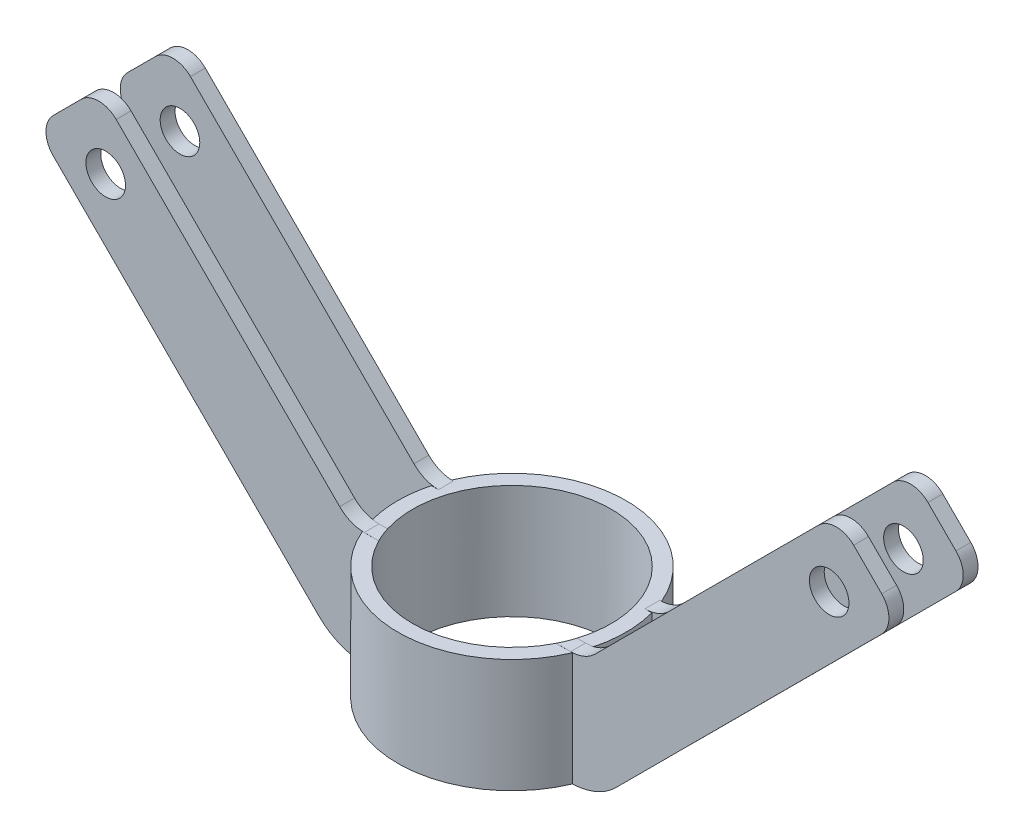
SolidWorks part; units mm, degrees
other "Objet de détail1"
other "Objet de détail2"
other "Objet de détail3"
other "Objet de détail4"
other "Objet de détail5"
other "Objet de détail6"
other "Dossier de soudure"
other "Cordon de soudure1"
other "Cordon de soudure2"
other "Cordon de soudure3"
other "Cordon de soudure4"
ref_plane "Plan de face" through (0, 0, 0) normal (0, 0, 1) x (1, 0, 0)
ref_plane "Plan de dessus" through (0, 0, 0) normal (0, 1, 0) x (1, 0, 0)
ref_plane "Plan de droite" through (0, 0, 0) normal (1, 0, 0) x (0, 0, -1)
sketch "Sketch1" plane through (0, 0, 0) normal (0, 0, 1) x (1, 0, 0)
  line L1 (0, 106.694) -> (0, -106.694) construction
  line L7 (-83.6899, 93.7758) -> (-30.0503, 40.1361)
  line L10 (20.8579, 36.3285) -> (-20.8579, 36.3285)
  line L11 (83.6899, 93.7758) -> (30.0503, 40.1361)
  line L12 (78.033, 106.5037) -> (83.6899, 100.8468)
  line L13 (25.8076, 61.3493) -> (70.9619, 106.5037)
  line L14 (-20.8579, 59.2991) -> (20.8579, 59.2991)
  line L15 (-25.8076, 61.3493) -> (-70.9619, 106.5037)
  line L16 (-78.033, 106.5037) -> (-83.6899, 100.8468)
  circle A4 centre (-73.0833, 95.8971) radius 4
  circle A5 centre (73.0833, 95.8971) radius 4
  arc A10 (-30.0503, 40.1361) -> (-20.8579, 36.3285) centre (-20.8579, 49.3285) ccw
  arc A11 (30.0503, 40.1361) -> (20.8579, 36.3285) centre (20.8579, 49.3285) cw
  arc A12 (83.6899, 93.7758) -> (83.6899, 100.8468) centre (80.1543, 97.3113) ccw
  arc A13 (78.033, 106.5037) -> (70.9619, 106.5037) centre (74.4975, 102.9681) ccw
  arc A14 (20.8579, 59.2991) -> (25.8076, 61.3493) centre (20.8579, 66.2991) ccw
  arc A15 (-25.8076, 61.3493) -> (-20.8579, 59.2991) centre (-20.8579, 66.2991) ccw
  arc A16 (-70.9619, 106.5037) -> (-78.033, 106.5037) centre (-74.4975, 102.9681) ccw
  arc A17 (-83.6899, 100.8468) -> (-83.6899, 93.7758) centre (-80.1543, 97.3113) ccw
extrude "Boss.-Extru.1" add sketch "Sketch1" along normal blind 3
ref_plane "Plan1" through (0, 0, -12) normal (0, 0, -1) x (-1, 0, 0)
sketch "Sketch2" plane through (0, 0, -12) normal (0, 0, -1) x (-1, 0, 0)
  line L1 (-0.007, 106.687) -> (-0.007, -106.7009) construction
  line L9 (-25.8146, 61.3424) -> (-70.9689, 106.4967)
  line L10 (-78.04, 106.4967) -> (-83.6968, 100.8399)
  line L11 (-83.6968, 93.7688) -> (-30.0572, 40.1292)
  line L12 (20.8509, 36.3216) -> (-20.8648, 36.3216)
  line L13 (83.6829, 93.7688) -> (30.0433, 40.1292)
  line L14 (78.0261, 106.4967) -> (83.6829, 100.8399)
  line L15 (25.8007, 61.3424) -> (70.955, 106.4967)
  line L16 (-20.8648, 59.2921) -> (20.8509, 59.2921)
  circle A4 centre (-73.0902, 95.8901) radius 4
  circle A5 centre (73.0763, 95.8901) radius 4
  arc A10 (-70.9689, 106.4967) -> (-78.04, 106.4967) centre (-74.5044, 102.9612) ccw
  arc A11 (-83.6968, 100.8399) -> (-83.6968, 93.7688) centre (-80.1613, 97.3043) ccw
  arc A12 (-30.0572, 40.1292) -> (-20.8648, 36.3216) centre (-20.8648, 49.3216) ccw
  arc A13 (30.0433, 40.1292) -> (20.8509, 36.3216) centre (20.8509, 49.3216) cw
  arc A14 (83.6829, 93.7688) -> (83.6829, 100.8399) centre (80.1474, 97.3043) ccw
  arc A15 (78.0261, 106.4967) -> (70.955, 106.4967) centre (74.4905, 102.9612) ccw
  arc A16 (20.8509, 59.2921) -> (25.8007, 61.3424) centre (20.8509, 66.2921) ccw
  arc A17 (-25.8146, 61.3424) -> (-20.8648, 59.2921) centre (-20.8648, 66.2921) ccw
extrude "Boss.-Extru.2" add sketch "Sketch2" along normal blind 3 separate body
sketch "Sketch3" plane through (0, 59.2921, 0) normal (0, 1, 0) x (1, 0, 0)
  line L0 (-0.0021, 5.3168) -> (0, 0) construction
  line L2 (-8.1178, 6) -> (6.7917, 6) construction
  circle A0 centre (-0.0021, 6) radius 20.05
  dimension "D2" = 40.1
sketch "Sketch5" plane through (0, 59.2921, 0) normal (0, 1, 0) x (1, 0, 0)
  line L0 (-0.0021, 22.0811) -> (-0.0021, -12.3278) construction
  circle A5 centre (-0.0021, 6) radius 20.05
  circle A6 centre (-0.0021, 6) radius 23.05
  dimension "D2" = 40.1
  dimension "D3" = 3
extrude "Cut-Extrude1" cut sketch "Sketch3" against normal through all and the other way blind 10
extrude "Boss.-Extru.3" add sketch "Sketch5" against normal up to surface (22.9706 mm away) up to face at (-19.7036, 36.3216, -13.5061)
